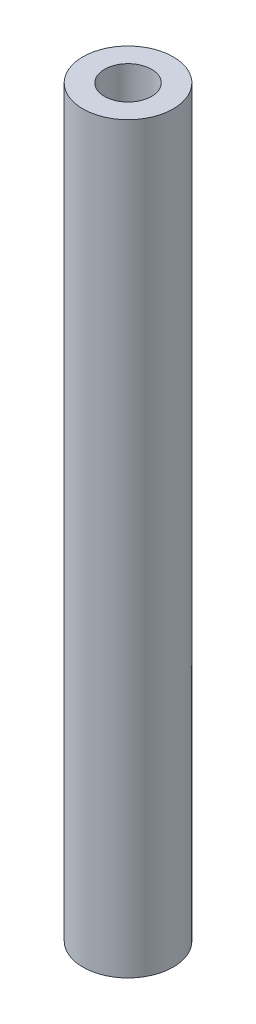
from build123d import *

# Parameters (mm, degrees)
F_25_0_25_DIAMETER_HOLE1_D     = 25
F_25_0_25_DIAMETER_HOLE1_DEPTH = 30
F_25_0_25_DIAMETER_HOLE1_TIP   = 7.510757738


with BuildPart() as part:
    # Sketch1 → Revolve1 (revolve)
    with BuildSketch(Plane(origin=(0, 0, 0), x_dir=(0, 0, -1), z_dir=(1, 0, 0))):
        Polygon((0, 395), (24, 395), (24, 0), (9.25, 0), (9.25, 5), (11.5, 5), (11.5, 8), (0, 8), align=None)
    revolve(axis=Axis((0, 0, 0), (0, 1, 0)))

    # Ø25.0 (25) Diameter Hole1
    with Locations(Plane.ZX.offset(395)):
        with Locations((0, 0)):
            Hole(F_25_0_25_DIAMETER_HOLE1_D / 2, depth=F_25_0_25_DIAMETER_HOLE1_DEPTH)
            with Locations((0, 0, -(F_25_0_25_DIAMETER_HOLE1_DEPTH + F_25_0_25_DIAMETER_HOLE1_TIP / 2))):  # 118° drill point
                Cone(0, F_25_0_25_DIAMETER_HOLE1_D / 2, F_25_0_25_DIAMETER_HOLE1_TIP, mode=Mode.SUBTRACT)


solid = part.part
